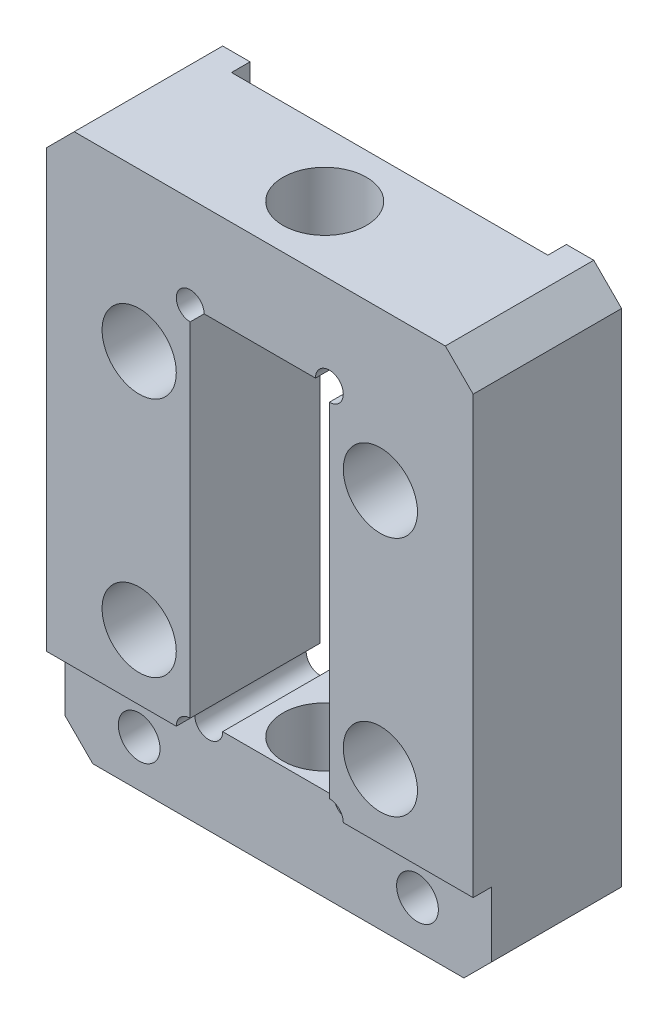
SolidWorks part; units mm, degrees
material "6061 合金"
ref_plane "前视基准面" through (0, 0, 0) normal (0, 0, 1) x (1, 0, 0)
ref_plane "上视基准面" through (0, 0, 0) normal (0, 1, 0) x (1, 0, 0)
ref_plane "右视基准面" through (0, 0, 0) normal (1, 0, 0) x (0, 0, -1)
sketch "草图1" plane through (0, 0, 0) normal (0, 0, 1) x (1, 0, 0)
  line L1 (-23, 30) -> (23, 30)
  line L2 (-23, 30) -> (-23, -30)
  line L3 (-23, -30) -> (23, -30)
  line L4 (23, 30) -> (23, -30)
  line L5 (-23, 30) -> (23, -30) construction
  line L6 (-23, -30) -> (23, 30) construction
  point P0 (0, 0)
  dimension "D1" = 60
  dimension "D2" = 46
extrude "凸台-拉伸1" add sketch "草图1" along normal mid plane 16
hole_wizard "M4 螺纹孔1" positions "草图8" profile "草图7" tap size "M4" standard "GB"
sketch "草图8" plane through (-23, 0, 0) normal (-1, 0, 0) x (0, 0, 1)
  line L0 (12.5, 30) -> (-12.5, 30) construction
  point P0 (0, 5)
  point P2 (0, -5)
  dimension "D1" = 25
  dimension "D2" = 10
sketch "草图7" plane through (-23, 5, 0) normal (0, 1, 0) x (0, 0, 1)
  line L0 (0, 0) -> (0, 13.0914)
  line L1 (0, 13.0914) -> (1.65, 12.1)
  line L2 (1.65, 12.1) -> (1.65, 0)
  line L5 (1.65, 0) -> (0, 0)
  line L10 (0, 13.0914) -> (-1.65, 12.1) construction
  line L11 (0, -6.35) -> (0, 107.95) construction
  dimension "螺纹孔钻头直径" = 3.3
  dimension "螺纹孔钻头深度" = 12.1
  dimension "导头角度" = 118
cosmetic thread "孔螺蚊线1" [suppressed] parameters "D1"=10, "D2"=4
cosmetic thread "孔螺蚊线2" [suppressed] parameters "D1"=10, "D2"=4
sketch "草图19" plane through (0, 0, 8) normal (0, 0, 1) x (1, 0, 0)
  line L1 (104.7133, -81.4109) -> (-38.2432, -81.4109)
  line L2 (104.7133, -81.4109) -> (104.7133, -20)
  line L3 (104.7133, -20) -> (-38.2432, -20)
  line L4 (-38.2432, -81.4109) -> (-38.2432, -20)
  line L5 (104.7133, -81.4109) -> (-38.2432, -20) construction
  line L6 (104.7133, -20) -> (-38.2432, -81.4109) construction
  line L7 (-23, -30) -> (23, -30) construction
  point P0 (33.235, -50.7054)
  dimension "D1" = 10
extrude "切除-拉伸7" cut sketch "草图19" against normal blind 2
sketch "草图21" plane through (0, 0, 8) normal (0, 0, 1) x (1, 0, 0)
  line L0 (23, 30) -> (-23, 30) construction
  line L1 (-7.5, 20) -> (7.5, 20)
  line L2 (-7.5, 20) -> (-7.5, -20)
  line L3 (-7.5, -20) -> (7.5, -20)
  line L4 (7.5, 20) -> (7.5, -20)
  line L5 (-7.5, 20) -> (7.5, -20) construction
  line L6 (-7.5, -20) -> (7.5, 20) construction
  line L8 (-23, -30) -> (23, -30) construction
  point P0 (0, 0)
  dimension "D1" = 10
  dimension "D2" = 15
  dimension "D3" = 10
extrude "切除-拉伸9" cut sketch "草图21" against normal through all
hole_wizard "Ø3.0 (3) 直径孔1" positions "草图23" profile "草图22" hole size "Ø3.0" standard "GB" end condition through all
sketch "草图23" plane through (0, 0, 8) normal (0, 0, 1) x (1, 0, 0)
  point P0 (-7.5, 20)
  point P3 (7.5, 20)
  point P6 (-7.5, -20)
  point P9 (7.5, -20)
sketch "草图22" plane through (-7.5, 20, 8) normal (1, 0, 0) x (0, -1, 0)
  line L0 (0, 0) -> (0, 16)
  line L1 (0, 16) -> (1.5, 16)
  line L2 (1.5, 16) -> (1.5, 0)
  line L5 (1.5, 0) -> (0, 0)
  line L11 (0, -6.35) -> (0, 107.95) construction
  dimension "通孔孔直径" = 3
  dimension "通孔孔深度" = 16
hole_wizard "Ø9.0 (9) 直径孔1" positions "草图25" profile "草图24" hole size "Ø9.0" standard "GB" end condition through all
sketch "草图25" plane through (0, 30, 0) normal (0, 1, 0) x (1, 0, 0)
  line L0 (23, 8) -> (-23, 8) construction
  point P0 (0, -1)
  dimension "D1" = 9
sketch "草图24" plane through (0, 30, 1) normal (1, 0, 0) x (0, 0, 1)
  line L0 (0, 0) -> (0, 60)
  line L1 (0, 60) -> (4.5, 60)
  line L2 (4.5, 60) -> (4.5, 0)
  line L5 (4.5, 0) -> (0, 0)
  line L11 (0, -6.35) -> (0, 107.95) construction
  dimension "通孔孔直径" = 9
  dimension "通孔孔深度" = 60
sketch "草图26" plane through (0, 0, -8) normal (0, 0, -1) x (-1, 0, 0)
  line L1 (-17.05, 42.2059) -> (17.05, 42.2059)
  line L2 (-17.05, 42.2059) -> (-17.05, -42.2059)
  line L3 (-17.05, -42.2059) -> (17.05, -42.2059)
  line L4 (17.05, 42.2059) -> (17.05, -42.2059)
  line L5 (-17.05, 42.2059) -> (17.05, -42.2059) construction
  line L6 (-17.05, -42.2059) -> (17.05, 42.2059) construction
  point P0 (0, 0)
  dimension "D1" = 34.1
extrude "切除-拉伸10" cut sketch "草图26" against normal blind 2
hole_wizard "打孔尺寸(%根据)开槽圆柱头螺钉的类型3" positions "草图14" profile "草图13" counterbore size "M4" standard "GB" end condition through all
sketch "草图14" plane through (0, 0, -8) normal (0, 0, -1) x (-1, 0, 0)
  line L0 (-15, -25) -> (15, -25) construction
  line L3 (0, -25) -> (0, 0) construction
  line L6 (-23, 30) -> (-17.05, 30) construction
  point P0 (-15, -25)
  point P2 (15, -25)
  dimension "D1" = 55
  dimension "D2" = 30
sketch "草图13" plane through (15, -25, -8) normal (1, 0, 0) x (0, 1, 0)
  line L0 (0, 0) -> (0, 16)
  line L1 (0, 16) -> (2.25, 16)
  line L3 (2.25, 16) -> (2.25, 7)
  line L4 (2.25, 7) -> (4, 7)
  line L5 (4, 7) -> (4, 0)
  line L7 (4, 0) -> (0, 0)
  line L11 (0, -6.35) -> (0, 107.95) construction
  dimension "通孔孔直径" = 4.5
  dimension "通孔孔深度" = 16
  dimension "柱形沉头孔直径" = 8
  dimension "柱形沉头孔深度" = 7
hole_wizard "打孔尺寸(%根据)开槽圆柱头螺钉的类型3" positions "草图3" profile "草图2" counterbore size "M4" standard "GB" end condition up to next
sketch "草图3" plane through (0, 0, 8) normal (0, 0, 1) x (1, 0, 0)
  line L0 (-13, 13) -> (13, 13) construction
  line L1 (13, 13) -> (13, -13) construction
  line L4 (0, 0) -> (0, 13) construction
  line L8 (-23, -30) -> (23, -30) construction
  point P0 (-13, 13)
  point P2 (13, 13)
  point P4 (-13, -13)
  point P6 (13, -13)
  dimension "D1" = 26
  dimension "D2" = 26
  dimension "D3" = 17
sketch "草图2" plane through (-13, 13, 8) normal (1, 0, 0) x (0, -1, 0)
  line L0 (0, 0) -> (0, 14)
  line L1 (0, 14) -> (2.1, 14)
  line L3 (2.1, 14) -> (2.1, 7)
  line L4 (2.1, 7) -> (4, 7)
  line L5 (4, 7) -> (4, 0)
  line L7 (4, 0) -> (0, 0)
  line L11 (0, -6.35) -> (0, 107.95) construction
  dimension "通孔孔直径" = 4.2
  dimension "通孔孔深度" = 14
  dimension "柱形沉头孔直径" = 8
  dimension "柱形沉头孔深度" = 7
chamfer "倒角2" distance 3 angle 45 2 edges at (23, 30, 0) (-23, 30, 0)
chamfer "倒角1" distance 3 angle 45 2 edges at (-23, -30, -1) (23, -30, -1)
sketch "草图30" plane through (0, 0, 8) normal (0, 0, 1) x (1, 0, 0)
  line L1 (60.6309, 39.6812) -> (-45.7176, 39.6812)
  line L2 (60.6309, 39.6812) -> (60.6309, 0)
  line L3 (60.6309, 0) -> (-45.7176, 0)
  line L4 (-45.7176, 39.6812) -> (-45.7176, 0)
  line L5 (60.6309, 39.6812) -> (-45.7176, 0) construction
  line L6 (60.6309, 0) -> (-45.7176, 39.6812) construction
  point P0 (7.4566, 19.8406)
extrude "切除-拉伸12" [suppressed] cut sketch "草图30" against normal blind 8
chamfer "倒角3" [suppressed] distance 8 angle 45
